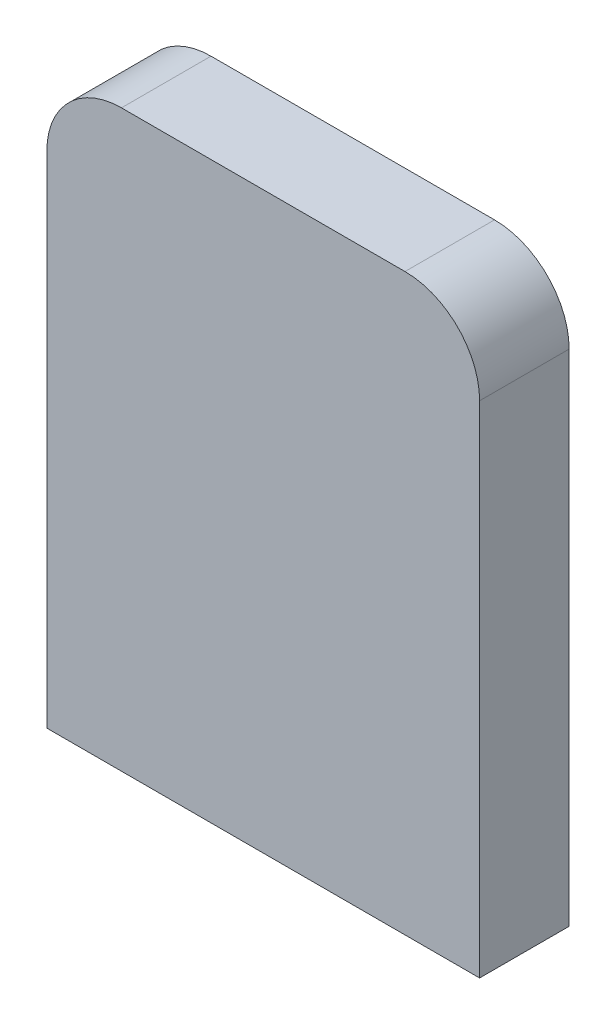
from build123d import *

# Parameters (mm, degrees)
SKETCH1_W           = 58
SKETCH1_H           = 77
BOSS_EXTRUDE1_DEPTH = 12
FILLET1_R           = 10


with BuildPart() as part:
    # Sketch1 → Boss-Extrude1 (new body)
    with BuildSketch(Plane.XY):
        Rectangle(SKETCH1_W, SKETCH1_H)
    extrude(amount=BOSS_EXTRUDE1_DEPTH)

    # Fillet1
    fillet1_edges = [part.edges().sort_by_distance(p)[0] for p in [
        (-29, 38.5, 6),
        (29, 38.5, 6),
    ]]
    fillet(fillet1_edges, radius=FILLET1_R)


solid = part.part
